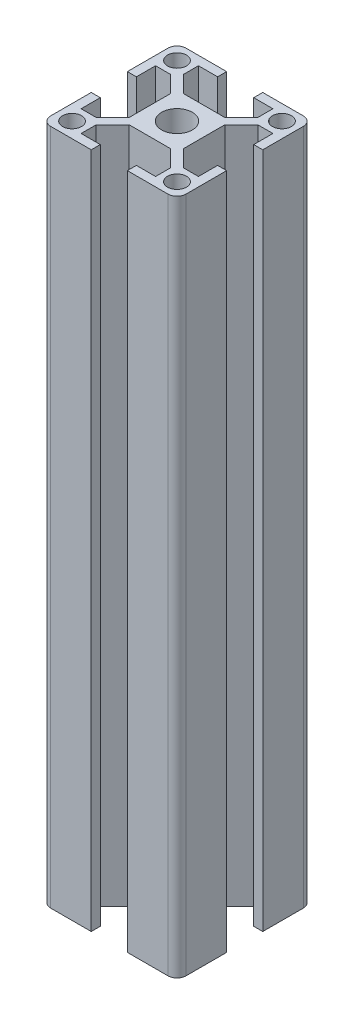
SolidWorks part; units mm, degrees
ref_plane "前视基准面" through (0, 0, 0) normal (0, 0, 1) x (1, 0, 0)
ref_plane "上视基准面" through (0, 0, 0) normal (0, 1, 0) x (1, 0, 0)
ref_plane "右视基准面" through (0, 0, 0) normal (1, 0, 0) x (0, 0, -1)
sketch "草图1" plane through (0, 0, 0) normal (0, 1, 0) x (1, 0, 0)
  line L44 (6.75, -28) -> (11, -28)
  line L45 (11, -28) -> (11, -30)
  line L46 (11, -30) -> (2, -30)
  line L47 (0, -28) -> (0, -19)
  line L48 (0, -19) -> (2, -19)
  line L49 (2, -19) -> (2, -23.25)
  line L50 (28, -30) -> (19, -30)
  line L51 (19, -30) -> (19, -28)
  line L52 (23.25, -28) -> (23.25, -24.6642)
  line L53 (19, -28) -> (23.25, -28)
  line L54 (30, -19) -> (30, -28)
  line L55 (28, -19) -> (30, -19)
  line L56 (28, -23.25) -> (28, -19)
  line L57 (24.6642, -23.25) -> (28, -23.25)
  line L58 (21, -19.5858) -> (24.6642, -23.25)
  line L59 (23.25, -24.6642) -> (19.5858, -21)
  line L60 (6.75, -24.6642) -> (6.75, -28)
  line L61 (2, -23.25) -> (5.3358, -23.25)
  line L62 (5.3358, -23.25) -> (9, -19.5858)
  line L63 (10.4142, -21) -> (6.75, -24.6642)
  line L64 (19.5858, -21) -> (10.4142, -21)
  line L65 (9, -19.5858) -> (9, -10.4142)
  line L66 (21, -10.4142) -> (21, -19.5858)
  line L67 (30, -11) -> (28, -11)
  line L68 (28, -11) -> (28, -6.75)
  line L69 (28, -6.75) -> (24.6642, -6.75)
  line L70 (24.6642, -6.75) -> (21, -10.4142)
  line L71 (19.5858, -9) -> (23.25, -5.3358)
  line L72 (10.4142, -9) -> (19.5858, -9)
  line L73 (6.75, -5.3358) -> (10.4142, -9)
  line L74 (9, -10.4142) -> (5.3358, -6.75)
  line L75 (2, -11) -> (0, -11)
  line L76 (2, -6.75) -> (2, -11)
  line L77 (5.3358, -6.75) -> (2, -6.75)
  line L78 (6.75, -2) -> (6.75, -5.3358)
  line L79 (23.25, -5.3358) -> (23.25, -2)
  line L80 (23.25, -2) -> (19, -2)
  line L81 (19, -2) -> (19, 0)
  line L82 (11, 0) -> (11, -2)
  line L83 (11, -2) -> (6.75, -2)
  line L84 (30, -2) -> (30, -11)
  line L85 (19, 0) -> (28, 0)
  line L86 (2, 0) -> (11, 0)
  line L87 (0, -11) -> (0, -2)
  line L88 (0, -15) -> (30, -15) construction
  line L89 (15, -30) -> (15, 0) construction
  line L90 (0, 0) -> (30, -30) construction
  line L91 (0, -30) -> (30, 0) construction
  arc A9 (0, -28) -> (2, -30) centre (2, -28) ccw
  circle A10 centre (3.375, -26.625) radius 2.1
  circle A11 centre (26.625, -26.625) radius 2.1
  arc A12 (28, -30) -> (30, -28) centre (28, -28) ccw
  circle A13 centre (15, -15) radius 3.4
  circle A14 centre (3.375, -3.375) radius 2.1
  circle A15 centre (26.625, -3.375) radius 2.1
  arc A16 (30, -2) -> (28, 0) centre (28, -2) ccw
  arc A17 (2, 0) -> (0, -2) centre (2, -2) ccw
  dimension "D2" = 15
  dimension "D5" = 6.8
  dimension "D8" = 6
  dimension "D11" = 23.25
  dimension "D12" = 3.375
  dimension "D13" = 23.25
  dimension "D14" = 4.2
  dimension "D15" = 2
  dimension "D16" = 2
  dimension "D23" = 2
  dimension "D24" = 2
  dimension "D1" = 15
  dimension "D3" = 45
  dimension "D4" = 45
  dimension "D6" = 30
  dimension "D7" = 30
  dimension "D9" = 12
  dimension "D10" = 3.375
  dimension "D17" = 11
  dimension "D18" = 8
  dimension "D19" = 2
  dimension "D20" = 2
  dimension "D21" = 11
  dimension "D22" = 8
  dimension "D25" = 2
  dimension "D26" = 2
  dimension "D27" = 6.75
  dimension "D28" = 16.5
  dimension "D29" = 6.75
  dimension "D30" = 16.5
  dimension "D31" = 12
  dimension "D32" = 6
  dimension "D33" = 2
  dimension "D34" = 1
  dimension "D35" = 2
  dimension "D36" = 1
extrude "拉伸1" add sketch "草图1" along normal blind 150
cosmetic thread "装饰螺纹线1" parameters "D1"=15, "D2"=8
